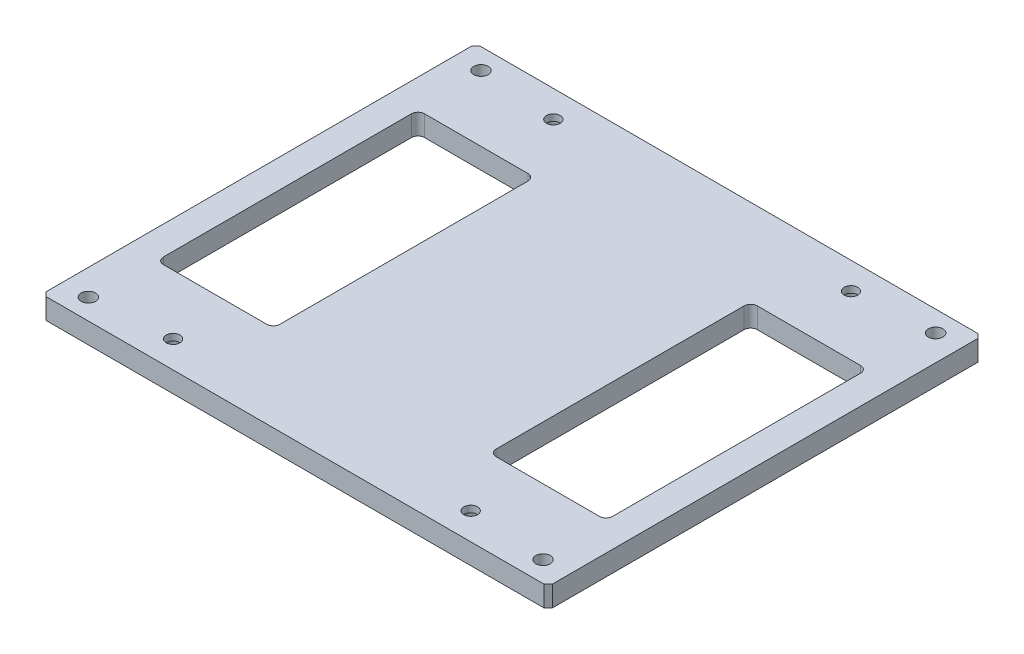
from build123d import *

# Parameters (mm, degrees)
SKETCH_1_W          = 245
SKETCH_1_H          = 210
EXTRUDE_1_DEPTH     = 10
CHAMFER_1_SIZE      = 2
CUT_EXTRUDE_1_REACH = 163.652
SKETCH_5_R          = 3.5
CUT_EXTRUDE_2_REACH = 163.652


with BuildPart() as part:
    # 草图1 → 凸台-拉伸1 (new body)
    with BuildSketch(Plane(origin=(0, 0, 0), x_dir=(1, 0, 0), z_dir=(0, 1, 0))):
        Rectangle(SKETCH_1_W, SKETCH_1_H)
    extrude(amount=EXTRUDE_1_DEPTH)

    # 倒角1
    chamfer_1_edges = [part.edges().sort_by_distance(p)[0] for p in [
        (122.5, 5, 105),
        (-122.5, 5, 105),
        (-122.5, 5, -105),
        (122.5, 5, -105),
    ]]
    chamfer(chamfer_1_edges, length=CHAMFER_1_SIZE)

    # 草图4 → 打孔尺寸(%根据)内六角圆柱头螺钉的类型1 (revolve, cut)
    with BuildSketch(Plane(origin=(72, 0, 92), x_dir=(0, 0, -1), z_dir=(1, 0, 0))):
        Polygon((0, 0), (0, 10.001), (3.3, 10.001), (3.3, 6.8), (5.5, 6.8), (5.5, 0.025), (5.525, 0), align=None)
    hole_wizard_1 = revolve(axis=Axis((72, -6.35, 92), (0, 1, 0)), mode=Mode.SUBTRACT)

    # 镜向1: 打孔尺寸(%根据)内六角圆柱头螺钉的类型1 across plane
    add(hole_wizard_1.mirror(Plane(origin=(0, 0, 0), x_dir=(0, 0, 1), z_dir=(1, 0, 0))), mode=Mode.SUBTRACT)

    # 镜向2: 打孔尺寸(%根据)内六角圆柱头螺钉的类型1 across plane
    add(hole_wizard_1.mirror(Plane.XY), mode=Mode.SUBTRACT)

    # 镜向2 copy 1 sketch → 镜向2 copy 1 (revolve, cut)
    with BuildSketch(Plane(origin=(-72, 0, -92), x_dir=(0, 0, 1), z_dir=(-1, 0, 0))):
        Polygon((0, 0), (0, 10.001), (3.3, 10.001), (3.3, 6.8), (5.5, 6.8), (5.5, 0.025), (5.525, 0), align=None)
    revolve(axis=Axis((-72, -6.35, -92), (0, 1, 0)), mode=Mode.SUBTRACT)

    # 草图5 → 切除-拉伸1 (cut, up to next)
    with BuildSketch(Plane(origin=(0, 10, 0), x_dir=(1, 0, 0), z_dir=(0, 1, 0)), mode=Mode.PRIVATE) as cut_extrude_1_sk1:
        with Locations(Location((-110, 95, 0), (0, 0, 270))):
            Circle(SKETCH_5_R)
    cut_extrude_1_tool1 = extrude(cut_extrude_1_sk1.sketch, amount=-CUT_EXTRUDE_1_REACH, mode=Mode.PRIVATE) & part.part
    # 草图5 → 切除-拉伸1 (cut, up to next)
    with BuildSketch(Plane(origin=(0, 10, 0), x_dir=(1, 0, 0), z_dir=(0, 1, 0)), mode=Mode.PRIVATE) as cut_extrude_1_sk2:
        with Locations(Location((110, 95, 0), (0, 0, 270))):
            Circle(SKETCH_5_R)
    cut_extrude_1_tool2 = extrude(cut_extrude_1_sk2.sketch, amount=-CUT_EXTRUDE_1_REACH, mode=Mode.PRIVATE) & part.part
    # 草图5 → 切除-拉伸1 (cut, up to next)
    with BuildSketch(Plane(origin=(0, 10, 0), x_dir=(1, 0, 0), z_dir=(0, 1, 0)), mode=Mode.PRIVATE) as cut_extrude_1_sk3:
        with Locations(Location((110, -95, 0), (0, 0, 270))):
            Circle(SKETCH_5_R)
    cut_extrude_1_tool3 = extrude(cut_extrude_1_sk3.sketch, amount=-CUT_EXTRUDE_1_REACH, mode=Mode.PRIVATE) & part.part
    # 草图5 → 切除-拉伸1 (cut, up to next)
    with BuildSketch(Plane(origin=(0, 10, 0), x_dir=(1, 0, 0), z_dir=(0, 1, 0)), mode=Mode.PRIVATE) as cut_extrude_1_sk4:
        with Locations(Location((-110, -95, 0), (0, 0, 270))):
            Circle(SKETCH_5_R)
    cut_extrude_1_tool4 = extrude(cut_extrude_1_sk4.sketch, amount=-CUT_EXTRUDE_1_REACH, mode=Mode.PRIVATE) & part.part
    add(cut_extrude_1_tool1.solids().sort_by_distance((-110, 10, -95))[0], mode=Mode.SUBTRACT)
    add(cut_extrude_1_tool2.solids().sort_by_distance((110, 10, -95))[0], mode=Mode.SUBTRACT)
    add(cut_extrude_1_tool3.solids().sort_by_distance((110, 10, 95))[0], mode=Mode.SUBTRACT)
    add(cut_extrude_1_tool4.solids().sort_by_distance((-110, 10, 95))[0], mode=Mode.SUBTRACT)

    # 草图6 → 切除-拉伸2 (cut, up to next)
    with BuildSketch(Plane(origin=(0, 10, 0), x_dir=(1, 0, 0), z_dir=(0, 1, 0)), mode=Mode.PRIVATE) as cut_extrude_2_sk1:
        with BuildLine():
            Line((105.5, -63.2), (55.5, -63.2))
            ThreePointArc((55.5, -63.2), (53.2372583, -62.2627417), (52.3, -60))
            Line((52.3, -60), (52.3, 60))
            ThreePointArc((52.3, 60), (53.2372583, 62.2627417), (55.5, 63.2))
            Line((55.5, 63.2), (105.5, 63.2))
            ThreePointArc((105.5, 63.2), (107.7627417, 62.2627417), (108.7, 60))
            Line((108.7, 60), (108.7, -60))
            ThreePointArc((108.7, -60), (107.7627417, -62.2627417), (105.5, -63.2))
        make_face()
    cut_extrude_2_tool1 = extrude(cut_extrude_2_sk1.sketch, amount=-CUT_EXTRUDE_2_REACH, mode=Mode.PRIVATE) & part.part
    cut_extrude_2 = cut_extrude_2_tool1.solids().sort_by_distance((80.5, 10, 0))[0]
    add(cut_extrude_2, mode=Mode.SUBTRACT)

    # 镜向3: 切除-拉伸2 across plane
    add(cut_extrude_2.mirror(Plane(origin=(0, 0, 0), x_dir=(0, 0, 1), z_dir=(1, 0, 0))), mode=Mode.SUBTRACT)


solid = part.part
